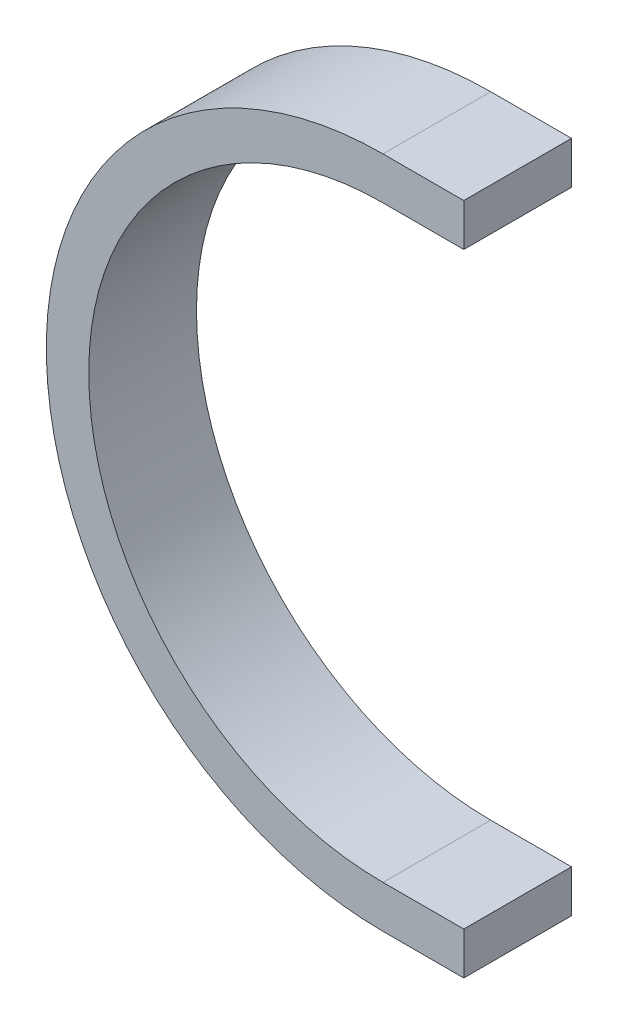
SolidWorks part; units mm, degrees
material "普通碳钢"
ref_plane "Front Plane" through (0, 0, 0) normal (0, 0, 1) x (1, 0, 0)
ref_plane "Top Plane" through (0, 0, 0) normal (0, 1, 0) x (1, 0, 0)
ref_plane "Right Plane" through (0, 0, 0) normal (1, 0, 0) x (0, 0, -1)
sketch "Sketch1" plane through (0, 0, 0) normal (0, 0, 1) x (1, 0, 0)
  line L0 (0, 79.375) -> (19.05, 79.375)
  line L1 (0, -79.375) -> (19.05, -79.375)
  line L2 (0, 69.375) -> (19.05, 69.375)
  line L3 (0, -69.375) -> (19.05, -69.375)
  line L4 (19.05, 79.375) -> (19.05, 69.375)
  line L5 (19.05, -69.375) -> (19.05, -79.375)
  arc A0 (0, 79.375) -> (0, -79.375) centre (0, 0) ccw
  arc A1 (0, 69.375) -> (0, -69.375) centre (0, 0) ccw
  dimension "D1" = 158.75
  dimension "D2" = 19.05
  dimension "D3" = 19.05
  dimension "D4" = 10
extrude "Boss-Extrude1" add sketch "Sketch1" along normal mid plane 25.4
